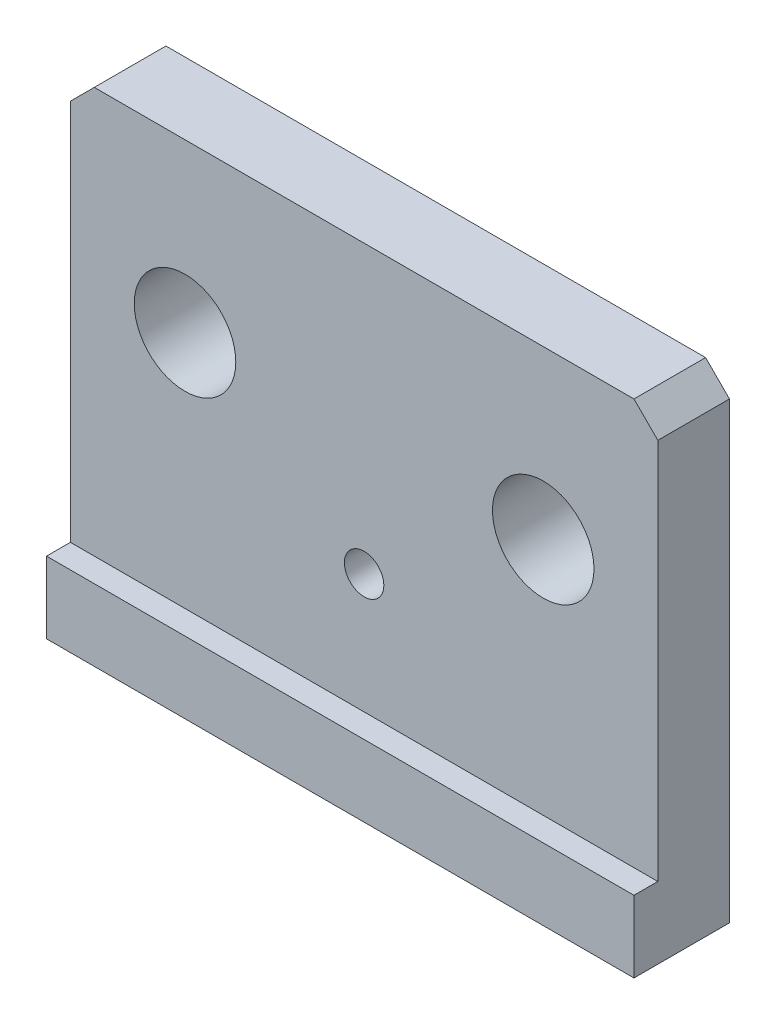
from build123d import *

# Parameters (mm, degrees)
SKETCH_1_W             = 49.2
SKETCH_1_H             = 40
EXTRUDE_1_DEPTH        = 8
HOLE_WIZARD_M4_1_D     = 3.3
HOLE_WIZARD_M4_1_DEPTH = 10.1
HOLE_WIZARD_M4_1_TIP   = 0.991420021
CHAMFER_1_SIZE         = 2
SKETCH_8_W             = 55.272888483
SKETCH_8_H             = 36.198084545
CUT_EXTRUDE_3_DEPTH    = 2
SKETCH_9_R             = 4.25
CUT_EXTRUDE_4_DEPTH    = 25
HOLE_WIZARD_M4_2_D     = 3.3
HOLE_WIZARD_M4_2_DEPTH = 10.1
HOLE_WIZARD_M4_2_TIP   = 0.991420021


with BuildPart() as part:
    # 草图1 → 凸台-拉伸1 (new body)
    with BuildSketch(Plane.XY):
        Rectangle(SKETCH_1_W, SKETCH_1_H)
    extrude(amount=EXTRUDE_1_DEPTH)

    # M4 螺纹孔1
    with Locations(Plane(origin=(0, -20, 0), x_dir=(-1, 0, 0), z_dir=(0, -1, 0))):
        with Locations((12.7, -4), (-12.7, -4)):
            Hole(HOLE_WIZARD_M4_1_D / 2, depth=HOLE_WIZARD_M4_1_DEPTH)
            with Locations((0, 0, -(HOLE_WIZARD_M4_1_DEPTH + HOLE_WIZARD_M4_1_TIP / 2))):  # 118° drill point
                Cone(0, HOLE_WIZARD_M4_1_D / 2, HOLE_WIZARD_M4_1_TIP, mode=Mode.SUBTRACT)

    # 倒角1
    chamfer_1_edges = [part.edges().sort_by_distance(p)[0] for p in [
        (-24.6, 20, 4),
        (24.6, 20, 4),
    ]]
    chamfer(chamfer_1_edges, length=CHAMFER_1_SIZE)

    # 草图8 → 切除-拉伸3 (cut)
    with BuildSketch(Plane.XY.offset(8)):
        with Locations((2.667874568, 4.099042273)):
            Rectangle(SKETCH_8_W, SKETCH_8_H)
    extrude(amount=-CUT_EXTRUDE_3_DEPTH, mode=Mode.SUBTRACT)

    # 草图9 → 切除-拉伸4 (cut)
    with BuildSketch(Plane(origin=(0, 0, 0), x_dir=(-1, 0, 0), z_dir=(0, 0, -1))):
        with Locations((-15, 6)):
            Circle(SKETCH_9_R)
        with Locations((15, 6)):
            Circle(SKETCH_9_R)
    extrude(amount=-CUT_EXTRUDE_4_DEPTH, mode=Mode.SUBTRACT)

    # M4 螺纹孔2
    with Locations(Plane.XY.offset(6)):
        with Locations((0, -4)):
            Hole(HOLE_WIZARD_M4_2_D / 2, depth=HOLE_WIZARD_M4_2_DEPTH)
            with Locations((0, 0, -(HOLE_WIZARD_M4_2_DEPTH + HOLE_WIZARD_M4_2_TIP / 2))):  # 118° drill point
                Cone(0, HOLE_WIZARD_M4_2_D / 2, HOLE_WIZARD_M4_2_TIP, mode=Mode.SUBTRACT)


solid = part.part
